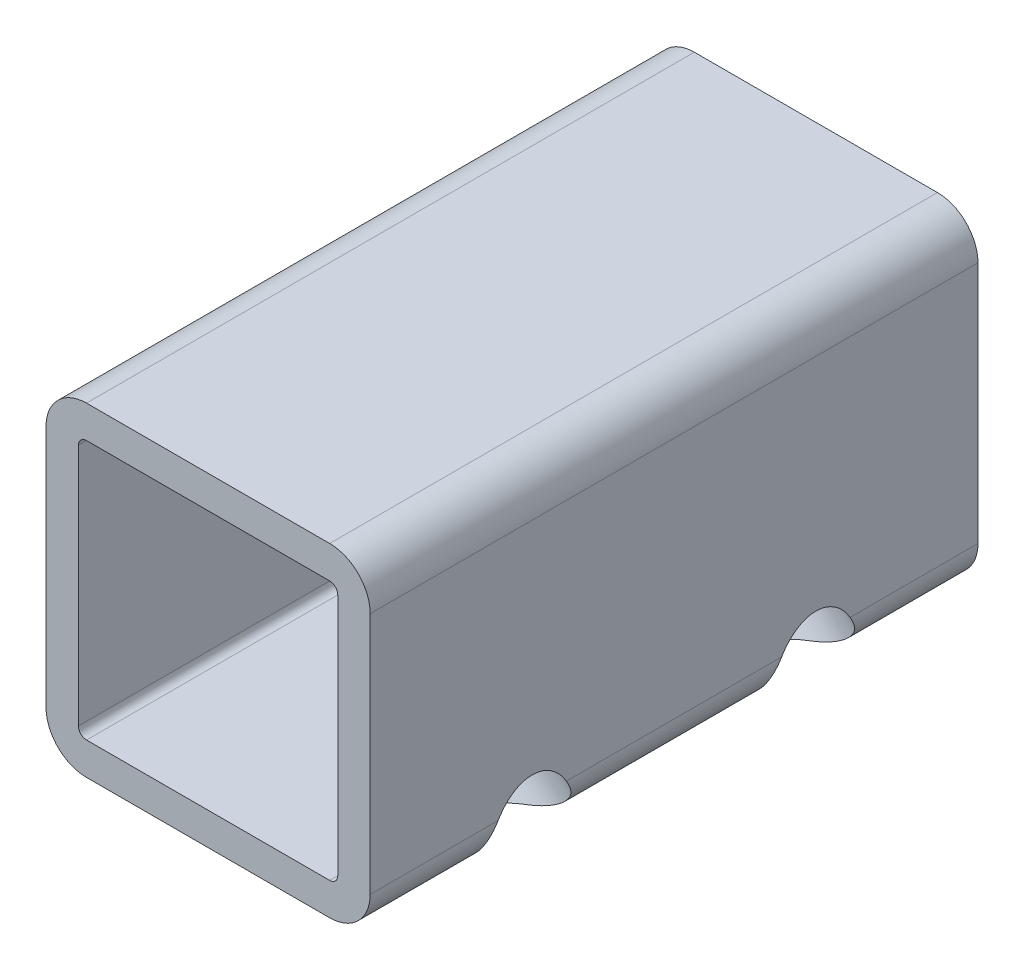
from build123d import *

# Parameters (mm, degrees)
BOSS_EXTRUDE1_DEPTH = 75
SKETCH2_R           = 5.5
CUT_EXTRUDE1_DEPTH  = 45


with BuildPart() as part:
    # Sketch1 → Boss-Extrude1 (new body)
    with BuildSketch(Plane.XY):
        with BuildLine():
            Line((-15, 20), (15, 20))
            ThreePointArc((15, 20), (18.535533906, 18.535533906), (20, 15))
            Line((20, 15), (20, -15))
            ThreePointArc((20, -15), (18.535533906, -18.535533906), (15, -20))
            Line((15, -20), (-15, -20))
            ThreePointArc((-15, -20), (-18.535533906, -18.535533906), (-20, -15))
            Line((-20, -15), (-20, 15))
            ThreePointArc((-20, 15), (-18.535533906, 18.535533906), (-15, 20))
        make_face()
        with BuildLine():
            Line((-15, 16), (15, 16))
            ThreePointArc((15, 16), (15.707106781, 15.707106781), (16, 15))
            Line((16, 15), (16, -15))
            ThreePointArc((16, -15), (15.707106781, -15.707106781), (15, -16))
            Line((15, -16), (-15, -16))
            ThreePointArc((-15, -16), (-15.707106781, -15.707106781), (-16, -15))
            Line((-16, -15), (-16, 15))
            ThreePointArc((-16, 15), (-15.707106781, 15.707106781), (-15, 16))
        make_face(mode=Mode.SUBTRACT)
    extrude(amount=BOSS_EXTRUDE1_DEPTH)

    # Sketch2 → Cut-Extrude1 (cut)
    with BuildSketch(Plane(origin=(0, 0, 0), x_dir=(0, 0, 1), z_dir=(-0.7071067811865476, 0.7071067811865475, 0))):
        with Locations(Location((20, 0, 0), (0, 0, 319.997252237))):
            Circle(SKETCH2_R)
        with Locations(Location((55, 0, 0), (0, 0, 220.002747763))):
            Circle(SKETCH2_R)
    extrude(amount=-CUT_EXTRUDE1_DEPTH, mode=Mode.SUBTRACT)


solid = part.part
